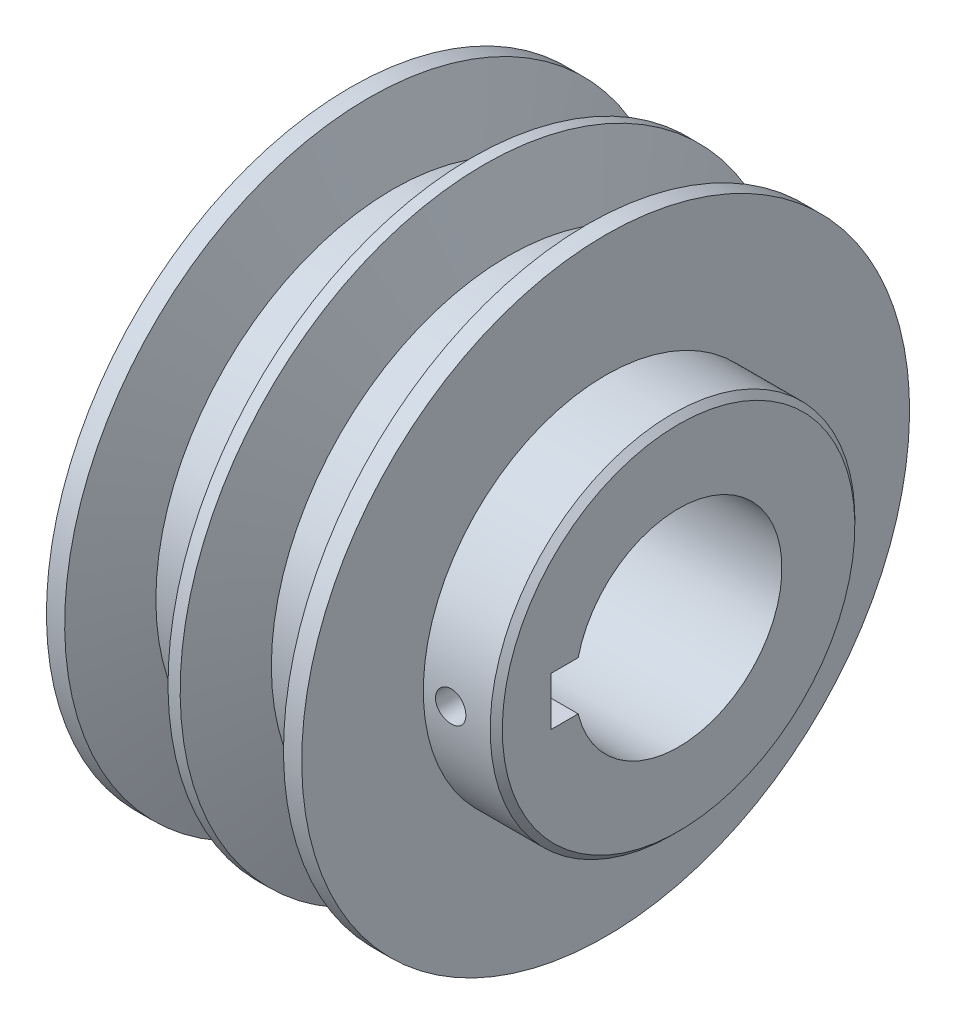
SolidWorks part; units mm, degrees
ref_plane "Front Plane" through (0, 0, 0) normal (0, 0, 1) x (1, 0, 0)
ref_plane "Top Plane" through (0, 0, 0) normal (0, 1, 0) x (1, 0, 0)
ref_plane "Right Plane" through (0, 0, 0) normal (1, 0, 0) x (0, 0, -1)
sketch "Sketch1" plane through (0, 0, 0) normal (0, 0, 1) x (1, 0, 0)
  line L0 (0, 0) -> (0, 50)
  line L1 (0, 50) -> (3, 50)
  line L2 (3, 50) -> (7.0037, 39)
  line L3 (7.0037, 39) -> (15.9963, 39)
  line L4 (15.9963, 39) -> (20, 50)
  line L5 (20, 50) -> (22, 50)
  line L6 (22, 50) -> (26.0037, 39)
  line L7 (26.0037, 39) -> (34.9963, 39)
  line L8 (34.9963, 39) -> (39, 50)
  line L9 (39, 50) -> (42, 50)
  line L10 (42, 50) -> (42, 30)
  line L11 (42, 30) -> (54, 30)
  line L12 (54, 30) -> (54, 0)
  line L13 (54, 0) -> (0, 0)
  line L14 (11.5, 52.8466) -> (11.5, 21.6016) construction
  line L15 (30.5, 54.4911) -> (30.5, 21.6016) construction
  dimension "D1" = 3
  dimension "D2" = 2
  dimension "D3" = 3
  dimension "D4" = 17
  dimension "D5" = 17
  dimension "D6" = 11
  dimension "D7" = 11
  dimension "D8" = 8.5
  dimension "D9" = 20
  dimension "D10" = 40
  dimension "D11" = 8.5
  dimension "D13" = 12
  dimension "D14" = 50
  dimension "D15" = 30
revolve "Revolve1" add sketch "Sketch1" angle 360 about L13
sketch "Sketch2" plane through (54, 0, 0) normal (1, 0, 0) x (0, 0, -1)
  circle A0 centre (0, 0) radius 17
  dimension "D1" = 34
extrude "Cut-Extrude1" cut sketch "Sketch2" against normal blind 70
hole_wizard "M6 Tapped Hole1" positions "Sketch6" profile "Sketch5" tap size "M6" standard "GB"
sketch "Sketch6" plane through (0, 0, 0) normal (0, 0, 1) x (1, 0, 0)
  line L0 (54, -30) -> (54, 30) construction
  point P2 (46.5, 0)
  dimension "D1" = 7.5
sketch "Sketch5" plane through (46.5, 0, 0) normal (1, 0, 0) x (0, 1, 0)
  line L0 (0, 0) -> (0, 51.5022)
  line L1 (0, 51.5022) -> (2.5, 50)
  line L2 (2.5, 50) -> (2.5, 0)
  line L5 (2.5, 0) -> (0, 0)
  line L10 (0, 51.5022) -> (-2.5, 50) construction
  line L11 (0, -6.35) -> (0, 107.95) construction
  dimension "螺纹孔钻头直径" = 5
  dimension "螺纹孔钻头深度" = 50
  dimension "导头角度" = 118
cosmetic thread "Hole thread 1" parameters "D1"=12, "D2"=6
chamfer "Chamfer1" distance 1 angle 45 1 edges at (54, 30, 0)
sketch "Sketch7" plane through (54, 0, 0) normal (1, 0, 0) x (0, 0, -1)
  line L1 (-21, -4) -> (-13, -4)
  line L2 (-21, -4) -> (-21, 4)
  line L3 (-21, 4) -> (-13, 4)
  line L4 (-13, -4) -> (-13, 4)
  line L5 (-21, -4) -> (-13, 4) construction
  line L6 (-21, 4) -> (-13, -4) construction
  circle A0 centre (0, 0) radius 17 construction
  point P0 (-17, 0)
  dimension "D1" = 8
  dimension "D2" = 8
extrude "Cut-Extrude2" cut sketch "Sketch7" against normal blind 70
